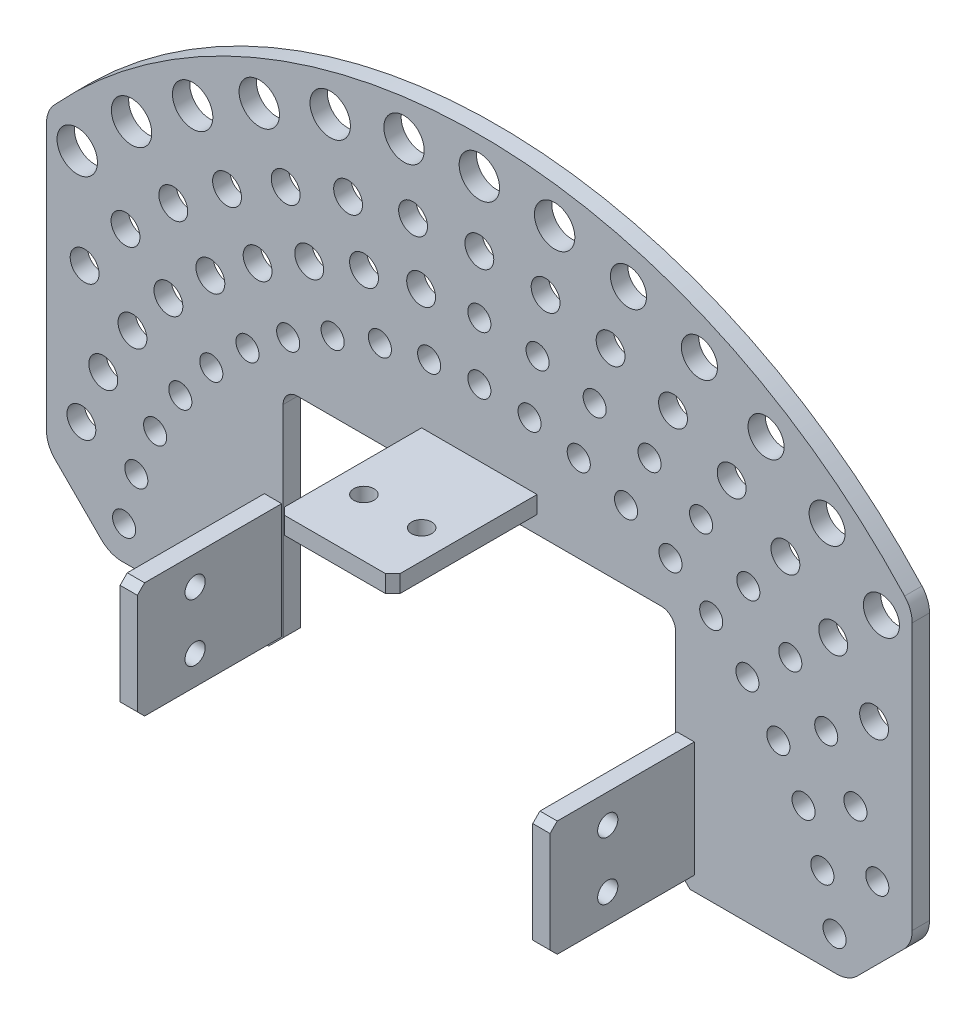
SolidWorks part; units mm, degrees
material "Q235-A "
ref_plane "前视基准面" through (0, 0, 0) normal (0, 0, 1) x (1, 0, 0)
ref_plane "上视基准面" through (0, 0, 0) normal (0, 1, 0) x (1, 0, 0)
ref_plane "右视基准面" through (0, 0, 0) normal (1, 0, 0) x (0, 0, -1)
sketch "草图1" plane through (0, 0, 0) normal (0, 0, 1) x (1, 0, 0)
  line L0 (0, 0) -> (0, 160)
  line L1 (0, 160) -> (272, 160)
  line L2 (272, 160) -> (272, 0)
  line L4 (136, 160) -> (136, -20) construction
  line L6 (0, 0) -> (-120, 0)
  line L7 (272, 0) -> (392, 0)
  line L8 (-120, 0) -> (-164, 44)
  line L9 (-164, 44) -> (-164, 244.5751)
  line L11 (436, 44) -> (436, 244.5751)
  line L12 (392, 0) -> (436, 44)
  arc A1 (436, 244.5751) -> (-164, 244.5751) centre (136, -20) ccw
  dimension "D2" = 120
  dimension "D5" = 800
  dimension "D1" = 272
  dimension "D3" = 160
  dimension "D4" = 45
  dimension "D6" = 600
  dimension "D7" = 20
extrude "凸台-拉伸1" add sketch "草图1" along normal blind 12
fillet "圆角1" radius 20 6 edges at (-120, 0, 6) (392, 0, 6) (436, 44, 6) (436, 244.5751, 6) (-164, 244.5751, 6) (-164, 44, 6)
fillet "圆角2" radius 10 2 edges at (0, 160, 6) (272, 160, 6)
sketch "草图2" plane through (0, 0, 12) normal (0, 0, 1) x (1, 0, 0)
  line L1 (-1, 90) -> (-13, 90)
  line L2 (-1, 90) -> (-1, 10)
  line L3 (-1, 10) -> (-13, 10)
  line L4 (-13, 90) -> (-13, 10)
  line L5 (136, 160) -> (136, -11.0693) construction
  line L6 (10, 160) -> (262, 160) construction
  line L7 (136, 160) -> (136, 172) construction
  line L20 (285, 90) -> (285, 10)
  line L21 (273, 10) -> (285, 10)
  line L22 (273, 90) -> (273, 10)
  line L23 (273, 90) -> (285, 90)
  line L32 (96, 172) -> (96, 184)
  line L33 (176, 172) -> (176, 184)
  line L34 (96, 184) -> (176, 184)
  line L35 (96, 172) -> (176, 172)
  line L36 (0, 0) -> (0, 150) construction
  dimension "D1" = 12
  dimension "D2" = 12
  dimension "D3" = 70
  dimension "D4" = 80
  dimension "D5" = 80
  dimension "D6" = 12
  dimension "D7" = 1
extrude "凸台-拉伸2" add sketch "草图2" along normal blind 100 separate body
sketch "草图3" plane through (-13, 0, 0) normal (-1, 0, 0) x (0, 0, 1)
  line L0 (112, 50) -> (31.461, 50) construction
  line L2 (112, 90) -> (112, 10) construction
  circle A0 centre (72, 70) radius 7
  circle A1 centre (72, 30) radius 7
  dimension "D1" = 14
  dimension "D3" = 40
  dimension "D2" = 40
extrude "切除-拉伸1" cut sketch "草图3" against normal through all
chamfer "倒角1" distance 5 angle 45 2 edges at (-7, 10, 112) (-7, 90, 112)
chamfer "倒角2" distance 5 angle 45 2 edges at (279, 10, 112) (279, 90, 112)
chamfer "倒角3" distance 5 angle 45 2 edges at (176, 178, 112) (96, 178, 112)
sketch "草图4" plane through (0, 184, 0) normal (0, 1, 0) x (1, 0, 0)
  line L0 (136, -112) -> (136, -12) construction
  line L1 (171, -112) -> (101, -112) construction
  line L2 (176, -12) -> (96, -12) construction
  line L3 (136, -72) -> (116, -72) construction
  circle A0 centre (116, -72) radius 7
  circle A1 centre (156, -72) radius 7
  dimension "D1" = 14
  dimension "D2" = 40
  dimension "D3" = 40
extrude "切除-拉伸2" cut sketch "草图4" against normal through all
sketch "草图5" plane through (0, 0, 12) normal (0, 0, 1) x (1, 0, 0)
  line L0 (136, -20) -> (136, 355) construction
  line L1 (136, -20) -> (188.1899, 351.3505) construction
  circle A0 centre (136, -20) radius 375 construction
  circle A1 centre (136, 355) radius 14
  circle A2 centre (188.1899, 351.3505) radius 14
  circle A3 centre (239.364, 340.4731) radius 14 construction
  circle A4 centre (288.5262, 322.5795) radius 14 construction
  circle A5 centre (334.7197, 298.018) radius 14 construction
  circle A6 centre (377.0454, 267.2667) radius 14 construction
  circle A7 centre (414.6793, 230.924) radius 14 construction
  circle A12 centre (-142.6793, 230.924) radius 14
  circle A13 centre (-105.0454, 267.2667) radius 14
  circle A14 centre (-62.7197, 298.018) radius 14
  circle A15 centre (-16.5262, 322.5795) radius 14
  circle A16 centre (32.636, 340.4731) radius 14
  circle A17 centre (83.8101, 351.3505) radius 14
  circle A18 centre (239.364, 340.4731) radius 12.5
  circle A19 centre (288.5262, 322.5795) radius 12.5
  circle A20 centre (334.7197, 298.018) radius 12.5
  circle A21 centre (377.0454, 267.2667) radius 12.5
  circle A22 centre (414.6793, 230.924) radius 12.5
  dimension "D1" = 750
  dimension "D2" = 28
  dimension "D5" = 25
  dimension "D4" = 8
  dimension "D3" = 7
extrude "切除-拉伸3" cut sketch "草图5" against normal through all
sketch "草图6" plane through (0, 0, 12) normal (0, 0, 1) x (1, 0, 0)
  line L0 (136, 380) -> (136, -20) construction
  line L1 (136, -20) -> (136, 310) construction
  line L2 (136, -20) -> (181.9271, 306.7885) construction
  arc A0 (430.7368, 250.4259) -> (-158.7368, 250.4259) centre (136, -20) ccw construction
  circle A1 centre (136, -20) radius 330 construction
  circle A2 centre (136, 310) radius 10
  circle A3 centre (181.9271, 306.7885) radius 10
  circle A4 centre (226.9603, 297.2164) radius 10
  circle A5 centre (270.2231, 281.47) radius 10
  circle A6 centre (310.8734, 259.8559) radius 10
  circle A7 centre (348.1199, 232.7947) radius 10
  circle A8 centre (381.2378, 200.8131) radius 10
  circle A9 centre (-109.2378, 200.8131) radius 10
  circle A10 centre (-76.1199, 232.7947) radius 10
  circle A11 centre (-38.8734, 259.8559) radius 10
  circle A12 centre (1.7769, 281.47) radius 10
  circle A13 centre (45.0397, 297.2164) radius 10
  circle A14 centre (90.0729, 306.7885) radius 10
  circle A15 centre (409.5824, 164.5337) radius 10
  circle A16 centre (-137.5824, 164.5337) radius 10
  dimension "D1" = 660
  dimension "D2" = 20
  dimension "D4" = 8
  dimension "D3" = 8
extrude "切除-拉伸4" cut sketch "草图6" against normal blind 50
sketch "草图7" plane through (0, 0, 12) normal (0, 0, 1) x (1, 0, 0)
  line L0 (136, 380) -> (136, -20) construction
  line L1 (136, -20) -> (136, 270) construction
  line L2 (136, -20) -> (176.3602, 267.1777) construction
  arc A0 (430.7368, 250.4259) -> (-158.7368, 250.4259) centre (136, -20) ccw construction
  circle A1 centre (136, -20) radius 290 construction
  circle A2 centre (136, 270) radius 8
  circle A3 centre (176.3602, 267.1777) radius 8
  circle A4 centre (215.9348, 258.7659) radius 8
  circle A5 centre (253.9536, 244.9282) radius 8
  circle A6 centre (289.6766, 225.9339) radius 8
  circle A7 centre (322.4084, 202.1529) radius 8
  circle A8 centre (351.512, 174.0479) radius 8
  circle A9 centre (376.4209, 142.1659) radius 8
  circle A10 centre (396.6503, 107.1276) radius 8
  circle A11 centre (411.8064, 69.6149) radius 8
  circle A12 centre (-139.8064, 69.6149) radius 8 construction
  circle A13 centre (-124.6503, 107.1276) radius 8 construction
  circle A14 centre (-104.4209, 142.1659) radius 8 construction
  circle A15 centre (-79.512, 174.0479) radius 8 construction
  circle A16 centre (-50.4084, 202.1529) radius 8 construction
  circle A17 centre (-17.6766, 225.9339) radius 8 construction
  circle A18 centre (18.0464, 244.9282) radius 8 construction
  circle A19 centre (56.0652, 258.7659) radius 8 construction
  circle A20 centre (95.6398, 267.1777) radius 8 construction
  circle A21 centre (95.6398, 267.1777) radius 10
  circle A22 centre (56.0652, 258.7659) radius 10
  circle A23 centre (18.0464, 244.9282) radius 10
  circle A24 centre (-17.6766, 225.9339) radius 10
  circle A25 centre (-50.4084, 202.1529) radius 10
  circle A26 centre (-79.512, 174.0479) radius 10
  circle A27 centre (-104.4209, 142.1659) radius 10
  circle A28 centre (-124.6503, 107.1276) radius 10
  circle A29 centre (-139.8064, 69.6149) radius 10
  dimension "D1" = 580
  dimension "D2" = 16
  dimension "D5" = 20
  dimension "D4" = 8
  dimension "D3" = 10
extrude "切除-拉伸5" cut sketch "草图7" against normal through all
sketch "草图8" plane through (0, 0, 12) normal (0, 0, 1) x (1, 0, 0)
  line L0 (136, 380) -> (136, -20) construction
  line L1 (136, -20) -> (136, 230) construction
  line L2 (136, -20) -> (170.7933, 227.567) construction
  arc A0 (430.7368, 250.4259) -> (-158.7368, 250.4259) centre (136, -20) ccw construction
  circle A1 centre (136, -20) radius 250 construction
  circle A2 centre (136, 230) radius 8
  circle A3 centre (170.7933, 227.567) radius 8
  circle A4 centre (204.9093, 220.3154) radius 8
  circle A5 centre (237.6842, 208.3864) radius 8
  circle A6 centre (268.4798, 192.012) radius 8
  circle A7 centre (296.6969, 171.5111) radius 8
  circle A8 centre (321.7862, 147.2827) radius 8
  circle A9 centre (343.2594, 119.7982) radius 8
  circle A10 centre (360.6985, 89.5928) radius 8
  circle A11 centre (373.7641, 57.2542) radius 8
  circle A12 centre (382.2019, 23.412) radius 8
  circle A13 centre (-110.2019, 23.412) radius 8
  circle A14 centre (-101.7641, 57.2542) radius 8
  circle A15 centre (-88.6985, 89.5928) radius 8
  circle A16 centre (-71.2594, 119.7982) radius 8
  circle A17 centre (-49.7862, 147.2827) radius 8
  circle A18 centre (-24.6969, 171.5111) radius 8
  circle A19 centre (3.5202, 192.012) radius 8
  circle A20 centre (34.3158, 208.3864) radius 8
  circle A21 centre (67.0907, 220.3154) radius 8
  circle A22 centre (101.2067, 227.567) radius 8
  dimension "D1" = 500
  dimension "D2" = 16
  dimension "D4" = 8
  dimension "D3" = 11
extrude "切除-拉伸6" cut sketch "草图8" against normal blind 50
chamfer "倒角4" distance 10 angle 45 2 edges at (272, 0, 6) (0, 0, 6)
